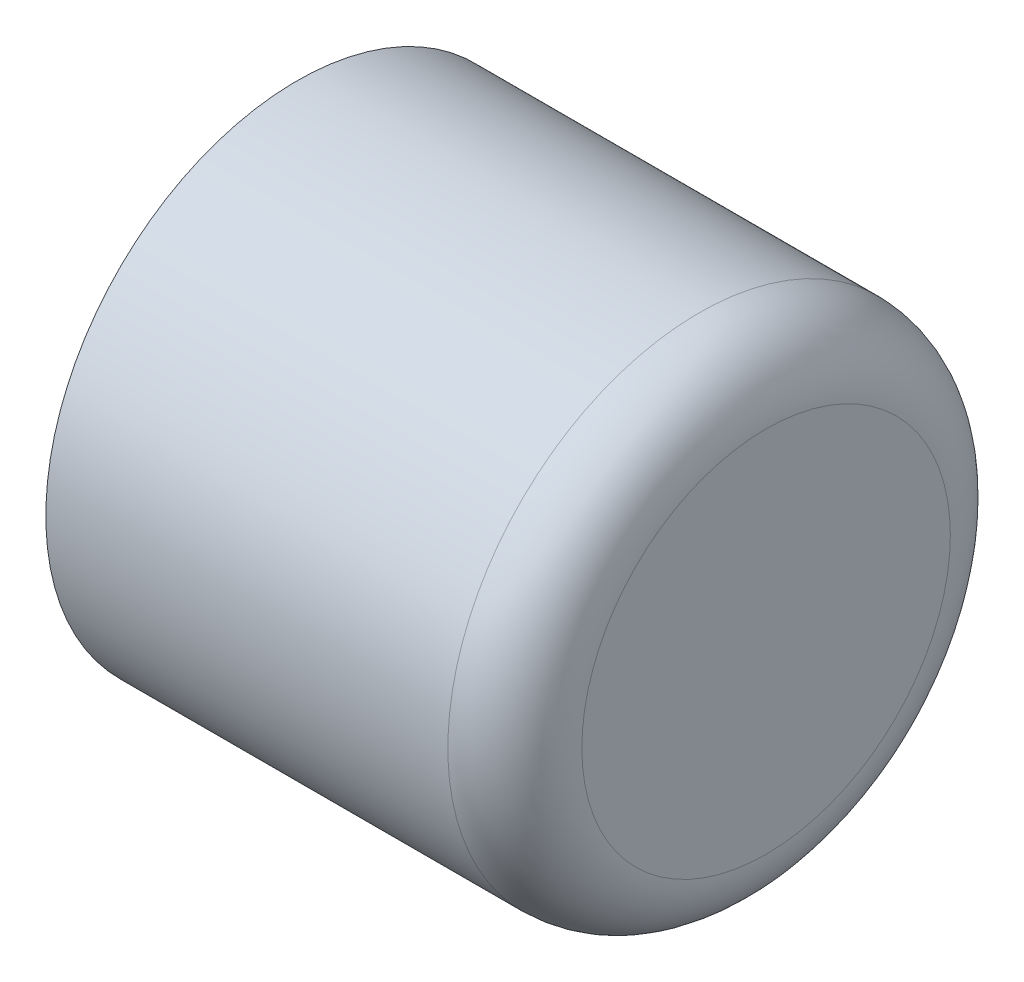
SolidWorks part; units mm, degrees
ref_plane "Front Plane" through (0, 0, 0) normal (0, 0, 1) x (1, 0, 0)
ref_plane "Top Plane" through (0, 0, 0) normal (0, 1, 0) x (1, 0, 0)
ref_plane "Right Plane" through (0, 0, 0) normal (1, 0, 0) x (0, 0, -1)
sketch "Sketch1" plane through (0, 0, 0) normal (0, 0, 1) x (1, 0, 0)
  line L0 (0, 0) -> (-13.4597, 0) construction
  line L1 (0, 0) -> (0, 5.5)
  line L2 (-2, 7.5) -> (-14, 7.5)
  line L3 (-14, 7.5) -> (-14, 4)
  line L4 (-14, 4) -> (-2.0171, 4)
  line L5 (-2.0171, 4) -> (-2.0171, 0)
  line L6 (-2.0171, 0) -> (0, 0)
  arc A0 (0, 5.5) -> (-2, 7.5) centre (-2, 5.5) ccw
  point P10 (0, 7.5)
  dimension "D5" = 2
  dimension "D1" = 7.5
  dimension "D2" = 3.5
  dimension "D3" = 14
  dimension "D4" = 4
revolve "Revolve1" add sketch "Sketch1" angle 360 about L0
